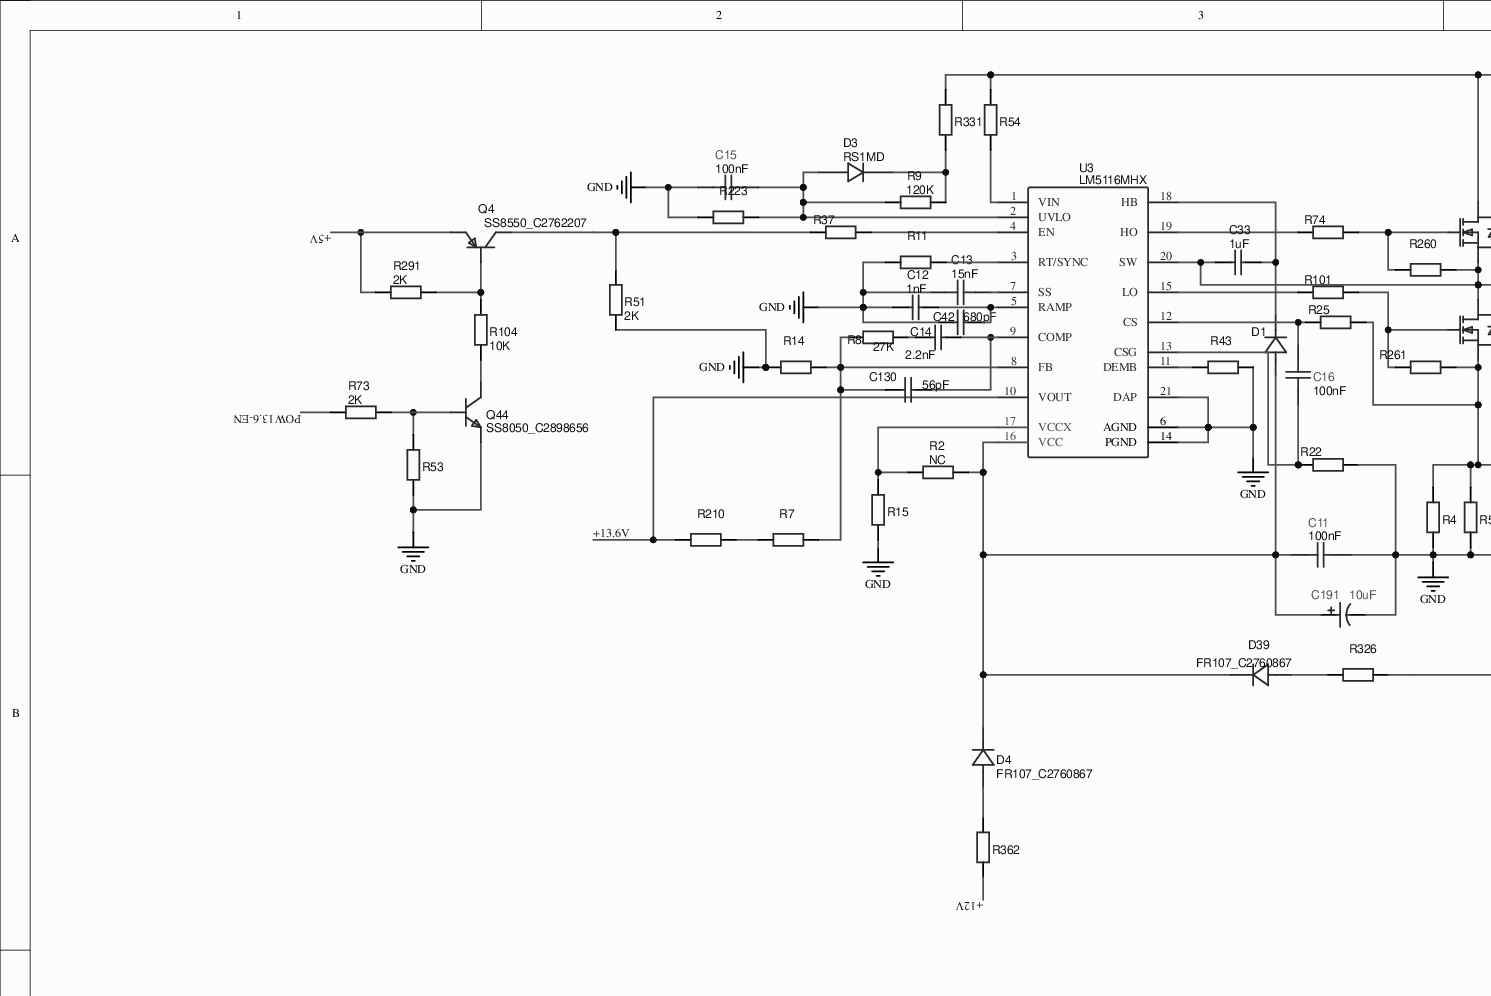
[diagram p0: MISC84402-12.SchDoc, top left]
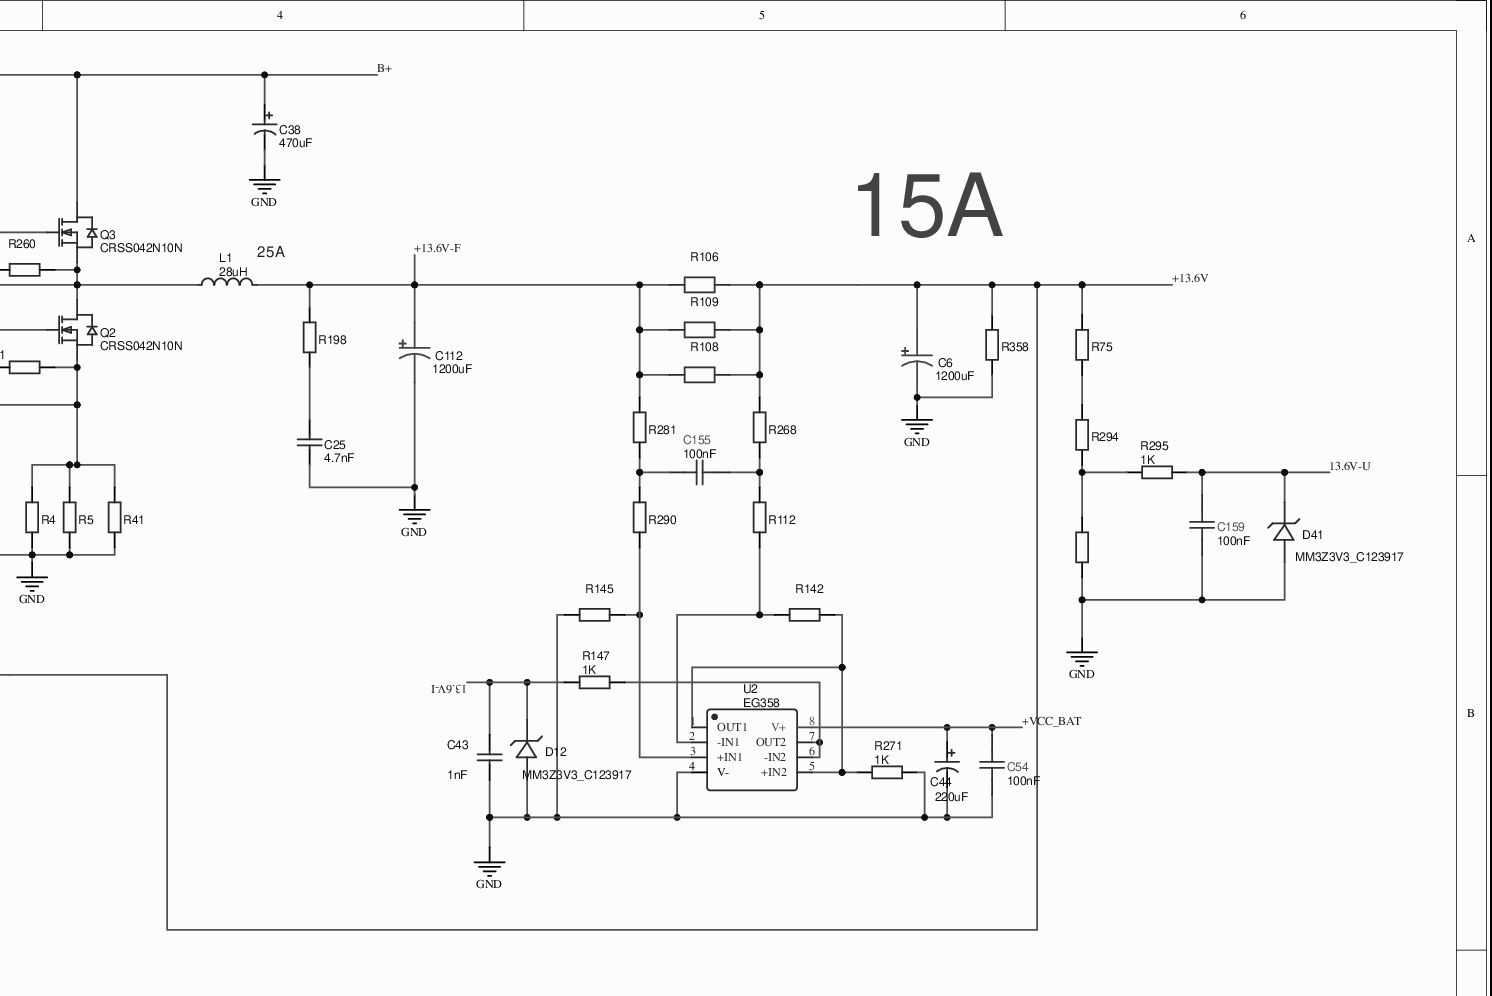
[diagram p1: MISC84402-12.SchDoc, top right]
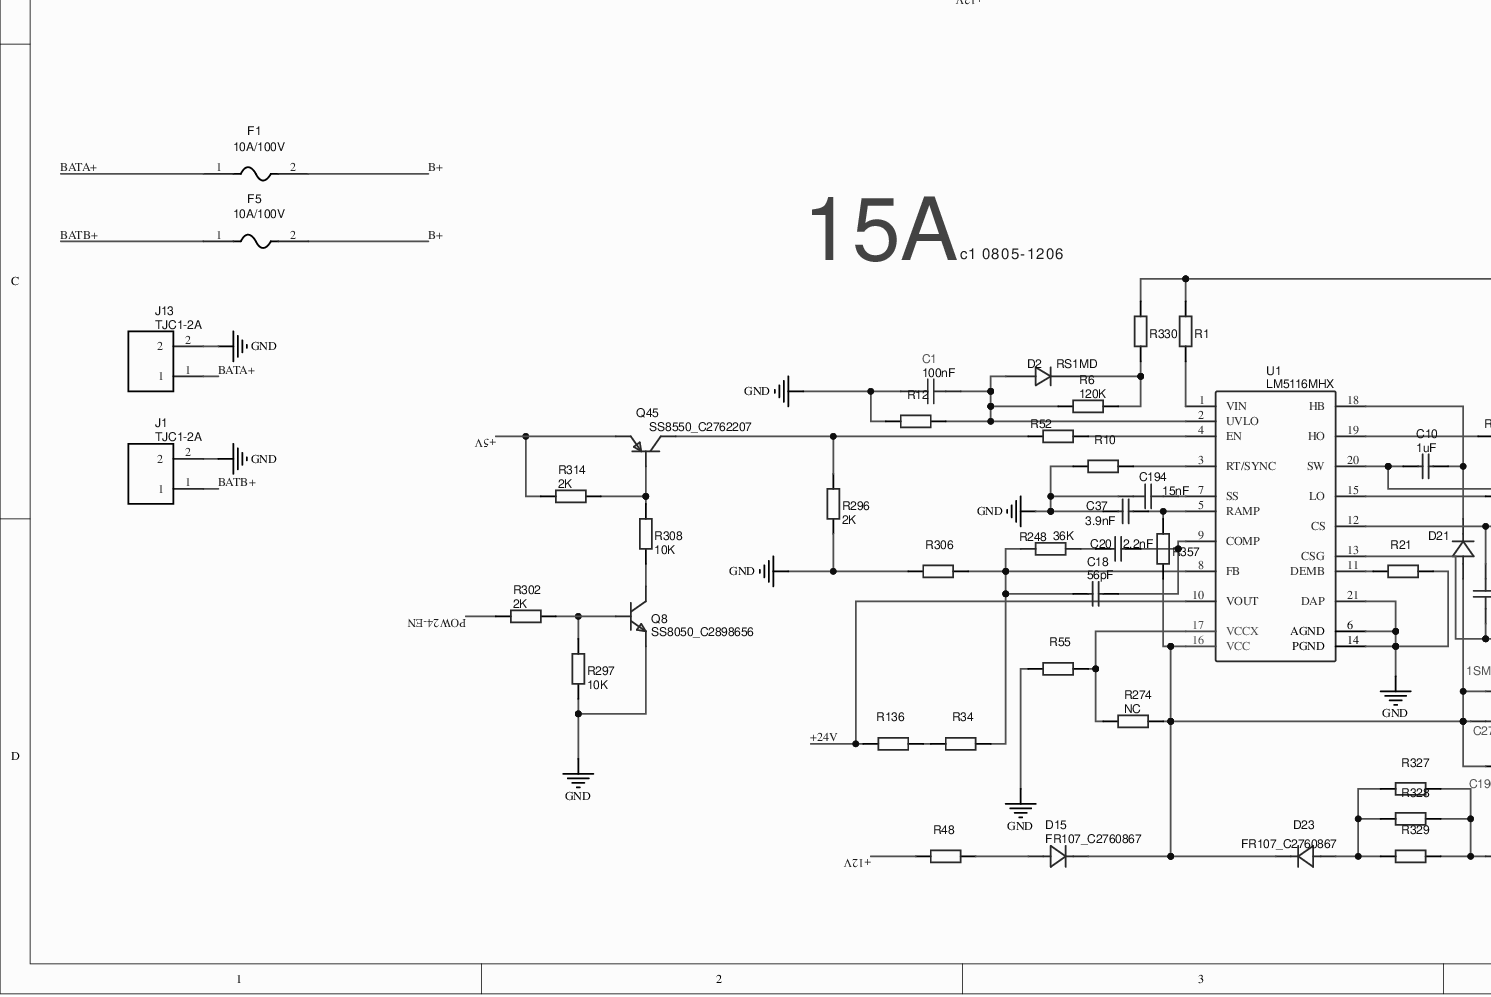
[diagram p2: MISC84402-12.SchDoc, bottom left]
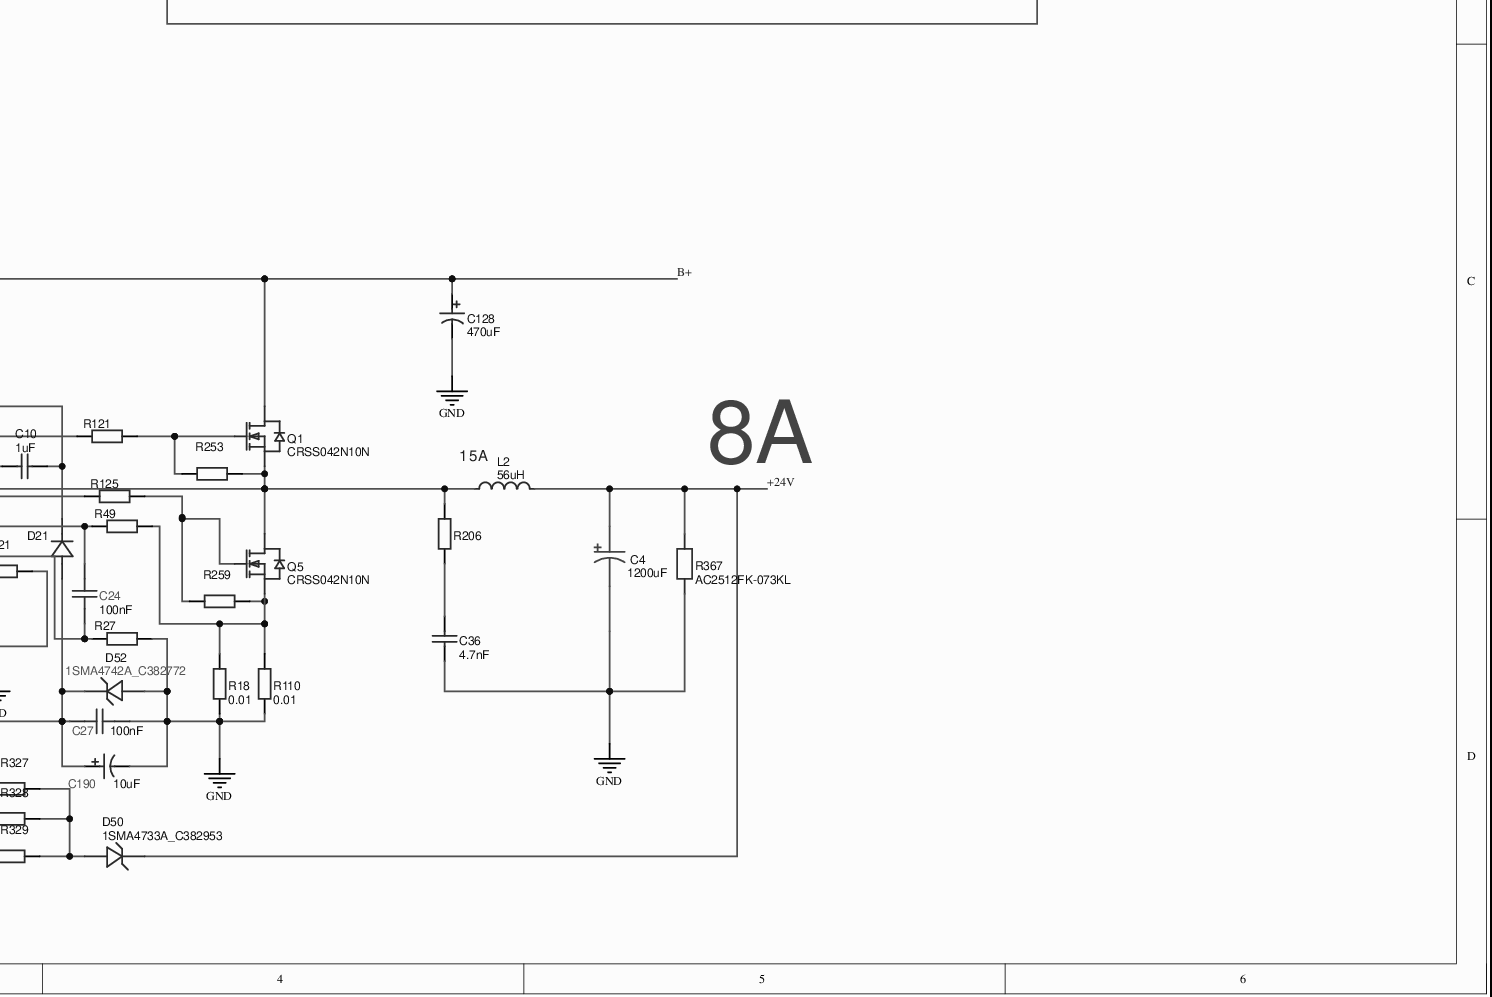
[diagram p3: MISC84402-12.SchDoc, bottom right]
# Altium project MISC84402-4.PrjPcb (part 4 of 7)

## Sheet MISC84402-12.SchDoc
size 488 x 321 mm

### Parts
C1  100nF  [C0603]
C4  1200uF  [CAP-TH_BD13.0-P5.00-D1.2-FD]
C6  1200uF  [CAP-TH_BD13.0-P5.00-D1.2-FD]
C10  1uF  [C0603]
C11  100nF  [C0603]
C12  1nF  [C0603]
C13  15nF  [C0603]
C14  2.2nF  [C0603]
C15  100nF  [C0603]
C16  100nF  [C0603]
C18  56pF  [C0603]
C20  2.2nF  [C0603]
C24  100nF  [C0603]
C25  4.7nF  [C1206]
C27  100nF  [C0603]
C33  1uF  [C0603]
C36  4.7nF  [C1206]
C37  3.9nF  [C0603]
C38  470uF  [CAP-TH_BD12.5-P5.00-D0.6-FD]
C42  680pF  [C0603]
C43  1nF  [C0603]
C44  220uF  [CAP-TH_BD6.3-P2.50-D1.0-FD]
C54  100nF  [C0603]
C112  1200uF  [CAP-TH_BD13.0-P5.00-D1.2-FD]
C128  470uF  [CAP-TH_BD12.5-P5.00-D0.6-FD]
C130  56pF  [C0603]
C155  100nF  [C0603]
C159  100nF  [C0603]
C190  10uF  [CAP-TH_BD5.0-P2.5-D0.5-FD]
C191  10uF  [CAP-TH_BD5.0-P2.5-D0.5-FD]
C194  15nF  [C0603]
D1  FR107_C2760867  [SOD-123FL_L2.7-W1.8-LS3.8-RD]  (value not drawn)
D2  RS1MD  [SMA_L4.3-W2.6-LS5.2-RD]
D3  RS1MD  [SMA_L4.3-W2.6-LS5.2-RD]
D4  FR107_C2760867  [SOD-123FL_L2.7-W1.8-LS3.8-RD]
D12  MM3Z3V3_C123917  [SOD-323_L1.8-W1.3-LS2.5-RD]
D15  FR107_C2760867  [SOD-123FL_L2.7-W1.8-LS3.8-RD]
D21  FR107_C2760867  [SOD-123FL_L2.7-W1.8-LS3.8-RD]  (value not drawn)
D23  FR107_C2760867  [SOD-123FL_L2.7-W1.8-LS3.8-RD]
D39  FR107_C2760867  [SOD-123FL_L2.7-W1.8-LS3.8-RD]
D41  MM3Z3V3_C123917  [SOD-323_L1.8-W1.3-LS2.5-RD]
D50  1SMA4733A_C382953  [SMA_L4.4-W2.6-LS5.0-RD]
D52  1SMA4742A_C382772  [SMA_L4.4-W2.6-LS5.0-RD]
F1  10A/100V  [FUSE-SMD_L6.1-W2.5]
F5  10A/100V  [FUSE-SMD_L6.1-W2.5]
J1  TJC1-2A  [CONN-TH_XT30UPB-F-W]
J13  TJC1-2A  [CONN-TH_XT30UPB-F-W]
L1  28uH  [IND-TH_CS270026-W280M-N]
L2  56uH  [IND-TH_CS270026-W560M-N]
Q1  CRSS042N10N  [TO-263-3_L10.2-W10.7-P5.08-LS16.2-TL]
Q2  CRSS042N10N  [TO-263-3_L10.2-W10.7-P5.08-LS16.2-TL]
Q3  CRSS042N10N  [TO-263-3_L10.2-W10.7-P5.08-LS16.2-TL]
Q4  SS8550_C2762207  [SOT-23-3_L2.9-W1.3-P1.90-LS2.4-BR]
Q5  CRSS042N10N  [TO-263-3_L10.2-W10.7-P5.08-LS16.2-TL]
Q8  SS8050_C2898656  [SOT-23-3_L2.9-W1.3-P1.90-LS2.4-BR]
Q44  SS8050_C2898656  [SOT-23-3_L2.9-W1.3-P1.90-LS2.4-BR]
Q45  SS8550_C2762207  [SOT-23-3_L2.9-W1.3-P1.90-LS2.4-BR]
R1  (no value)  [R1206]
R2  NC  [R0603]
R4  (no value)  [R2512]
R5  (no value)  [R2512]
R6  120K  [R0603]
R7  (no value)  [R0603]
R8  27K  [R0603]
R9  120K  [R0603]
R10  (no value)  [R0603]
R11  (no value)  [R0603]
R12  (no value)  [R0603]
R14  (no value)  [R0603]
R15  (no value)  [R0603]
R18  0.01  [R2512]
R21  (no value)  [R0603]
R22  (no value)  [R0603]
R25  (no value)  [R0603]
R27  (no value)  [R0603]
R34  (no value)  [R0603]
R37  (no value)  [R0603]
R41  (no value)  [R2512]
R43  (no value)  [R0603]
R48  (no value)  [R0603]
R49  (no value)  [R0603]
R51  2K  [R0603]
R52  (no value)  [R0603]
R53  (no value)  [R0603]
R54  (no value)  [R1206]
R55  (no value)  [R0603]
R73  2K  [R0603]
R74  (no value)  [R0805]
R75  (no value)  [R0603]
R101  (no value)  [R0805]
R104  10K  [R0603]
R106  (no value)  [R2512]
R107  (no value)  [R0603]
R108  (no value)  [R2512]
R109  (no value)  [R2512]
R110  0.01  [R2512]
R112  (no value)  [R0603]
R121  (no value)  [R0805]
R125  (no value)  [R0805]
R136  (no value)  [R0603]
R142  (no value)  [R0603]
R145  (no value)  [R0603]
R147  1K  [R0603]
R198  (no value)  [R1206]
R206  (no value)  [R1206]
R210  (no value)  [R0603]
R223  (no value)  [R0603]
R248  36K  [R0603]
R253  (no value)  [R0603]
R259  (no value)  [R0603]
R260  (no value)  [R0603]
R261  (no value)  [R0603]
R268  (no value)  [R0603]
R271  1K  [R0603]
R274  NC  [R0603]
R281  (no value)  [R0603]
R290  (no value)  [R0603]
R291  2K  [R0603]
R294  (no value)  [R0603]
R295  1K  [R0603]
R296  2K  [R0603]
R297  10K  [R0603]
R302  2K  [R0603]
R306  (no value)  [R0603]
R308  10K  [R0603]
R314  2K  [R0603]
R326  (no value)  [R0603]
R327  (no value)  [R0805]
R328  (no value)  [R0805]
R329  (no value)  [R0805]
R330  (no value)  [R1206]
R331  (no value)  [R1206]
R357  (no value)  [R0603]
R358  (no value)  [R2512]
R362  (no value)  [R0603]
R367  AC2512FK-073KL  [R2512]
U1  LM5116MHX  [HTSSOP-20_L6.5-W4.4-P0.65-LS6.4-BL-EP]
U2  EG358  [SOIC-8_L5.0-W4.0-P1.27-LS6.0-BL]
U3  LM5116MHX  [HTSSOP-20_L6.5-W4.4-P0.65-LS6.4-BL-EP]

### Nets
GND: C1.2 C4.2 C6.2 C11.1 C12.1 C13.2 C15.2 C25.1 C27.1 C36.1 C37.2 C38.2 C42.1 C43.1 C44.2 C54.2 C112.2 C128.2 C159.2 C190.2 C191.2 C194.2 D12.2(A) D41.2(A) D52.2(A) J1.2 J13.2 Q8.2(E) Q44.2(E) R4.1 R5.1 R10.1 R11.1 R12.1 R14.2 R15.1 R18.1 R21.2 R22.1 R27.1 R41.1 R43.2 R51.1 R53.2 R55.1 R107.1 R110.1 R145.1 R223.1 R271.2 R296.1 R297.2 R306.2 R358.1 R367.1 U1.6(AGND) U1.14(PGND) U1.21(DAP) U2.4(V-) U3.6(AGND) U3.14(PGND) U3.21(DAP)
13.6V-I: C43.2 D12.1(K) R147.2
13.6V-U: C159.1 D41.1(K) R295.1
+5V: Q4.2(E) Q45.2(E) R291.1 R314.1
+12V: R48.2 R362.1
+13.6V: C6.1 R75.2 R106.2 R108.2 R109.2 R210.1 R268.1 R326.2 R358.2 U3.10(VOUT)
+13.6V-F: C112.1 L1.2 R106.1 R108.1 R109.1 R198.2 R281.1
+24V: C4.1 D50.1(C) L2.2 R136.2 R367.2 U1.10(VOUT)
+VCC_BAT: C44.1 C54.1 U2.8(V+)
B+: C38.1 C128.1 F1.2 F5.2 Q1.2(D) Q3.2(D) R1.2 R54.2 R330.2 R331.2
BATA+: F1.1 J13.1
BATB+: F5.1 J1.1
POW13.6-EN: R73.1
POW24-EN: R302.1
NetC1_1: C1.1 D2.2 R6.1 R12.2 U1.2(UVLO)
NetC10_1: C10.1 L2.1 Q1.3(S) Q5.2(D) R206.2 R253.1 U1.20(SW)
NetC10_2: C10.2 D21.1(K) U1.18(HB)
NetC11_2: C11.2 C191.1 D1.2(A) D4.1(K) D39.1(K) R2.2 U3.16(VCC)
NetC12_2: C12.2 C42.2 U3.5(RAMP)
NetC13_1: C13.1 U3.7(SS)
NetC14_1: C14.1 R8.2
NetC14_2: C14.2 C130.1 U3.9(COMP)
NetC15_1: C15.1 D3.2 R9.1 R223.2 U3.2(UVLO)
NetC16_1: C16.1 R25.2 U3.12(CS)
NetC16_2: C16.2 R22.2 U3.13(CSG)
NetC18_1: C18.1 C20.1 U1.9(COMP)
NetC18_2: C18.2 R34.2 R248.1 R306.1 U1.8(FB)
NetC20_2: C20.2 R248.2
NetC24_1: C24.1 R49.2 U1.12(CS)
NetC24_2: C24.2 R27.2 U1.13(CSG)
NetC25_2: C25.2 R198.1
NetC27_2: C27.2 C190.1 D15.1(K) D21.2(A) D23.1(K) D52.1(C) R274.2 R357.1 U1.16(VCC)
NetC33_1: C33.1 L1.1 Q2.2(D) Q3.3(S) R260.1 U3.20(SW)
NetC33_2: C33.2 D1.1(K) U3.18(HB)
NetC36_2: C36.2 R206.1
NetC37_1: C37.1 R357.2 U1.5(RAMP)
NetC130_2: C130.2 R7.2 R8.1 R14.1 U3.8(FB)
NetC155_1: C155.1 R112.1 R268.2
NetC155_2: C155.2 R281.2 R290.1
NetC194_1: C194.1 U1.7(SS)
NetD2_1: D2.1 R6.2 R330.1
NetD3_1: D3.1 R9.2 R331.1
NetD4_2: D4.2(A) R362.2
NetD15_2: D15.2(A) R48.1
NetD23_2: D23.2(A) R327.1 R328.1 R329.1
NetD39_2: D39.2(A) R326.1
NetD50_2: D50.2(A) R327.2 R328.2 R329.2
NetQ1_1: Q1.1(G) R121.1 R253.2
NetQ2_1: Q2.1(G) R101.1 R261.2
NetQ2_3: Q2.3(S) R4.2 R5.2 R25.1 R41.2 R261.1
NetQ3_1: Q3.1(G) R74.1 R260.2
NetQ4_1: Q4.1(B) R104.2 R291.2
NetQ4_3: Q4.3(C) R37.1 R51.2
NetQ5_1: Q5.1(G) R125.1 R259.2
NetQ5_3: Q5.3(S) R18.2 R49.1 R110.2 R259.1
NetQ8_1: Q8.1(B) R297.1 R302.2
NetQ8_3: Q8.3(C) R308.1
NetQ44_1: Q44.1(B) R53.1 R73.2
NetQ44_3: Q44.3(C) R104.1
NetQ45_1: Q45.1(B) R308.2 R314.2
NetQ45_3: Q45.3(C) R52.1 R296.2
NetR1_1: R1.1 U1.1(VIN)
NetR2_1: R2.1 R15.2 U3.17(VCCX)
NetR7_1: R7.1 R210.2
NetR10_2: R10.2 U1.3(RT/SYNC)
NetR11_2: R11.2 U3.3(RT/SYNC)
NetR21_1: R21.1 U1.11(DEMB)
NetR34_1: R34.1 R136.1
NetR37_2: R37.2 U3.4(EN)
NetR43_1: R43.1 U3.11(DEMB)
NetR52_2: R52.2 U1.4(EN)
NetR54_1: R54.1 U3.1(VIN)
NetR55_2: R55.2 R274.1 U1.17(VCCX)
NetR74_2: R74.2 U3.19(HO)
NetR75_1: R75.1 R294.2
NetR101_2: R101.2 U3.15(LO)
NetR107_2: R107.2 R294.1 R295.2
NetR112_2: R112.2 R142.1 U2.2(-IN1)
NetR121_2: R121.2 U1.19(HO)
NetR125_2: R125.2 U1.15(LO)
NetR142_2: R142.2 R271.1 U2.1(OUT1) U2.5(+IN2)
NetR145_2: R145.2 R290.2 U2.3(+IN1)
NetR147_1: R147.1 U2.6(-IN2) U2.7(OUT2)

### Notes on the sheet
- (near L1) 25A
- 15A
- c1 0805-1206
- (near L2) 15A
- 8A

### Library data of the parts
C1 C11 C15 C16 C24 C27 C54 C155 C159 = 100nF: BOM_Manufacturer: SAMSUNG; BOM_Manufacturer Part: CL10B104KC8NNNC; nameAlias: Capacitance; BOM_Supplier: LCSC; BOM_Supplier Part: C15725; BOM_JLCPCB Part Class: Extended Part; spicePre: C; spiceSymbolName: CL10B104KC8NNNC
C4 C6 C112 = 1200uF: BOM_Manufacturer: CapXon; BOM_Manufacturer Part: GF122M025I200A; nameAlias: Capacitance; BOM_Supplier: LCSC; BOM_Supplier Part: C89779; BOM_JLCPCB Part Class: Extended Part; spicePre: C; spiceSymbolName: GF122M025I200A
C10 C33 = 1uF: BOM_Manufacturer Part: CL10A105KB8NNNC; BOM_Manufacturer: SAMSUNG; nameAlias: Capacitance; BOM_Supplier: LCSC; BOM_Supplier Part: C15849; BOM_JLCPCB Part Class: Basic Part; spicePre: C; spiceSymbolName: CL10A105KB8NNNC
C12 C43 = 1nF: BOM_Manufacturer Part: CL10B102KB8NNNC; BOM_Manufacturer: SAMSUNG; nameAlias: Capacitance; BOM_Supplier: LCSC; BOM_Supplier Part: C1588; BOM_JLCPCB Part Class: Basic Part; spicePre: C; spiceSymbolName: CL10B102KB8NNNC
C13 C194 = 15nF: BOM_Manufacturer: Walsin Tech Corp; BOM_Manufacturer Part: 0603B153K500CT; nameAlias: Capacitance; Contributor: LCSC; BOM_Supplier: LCSC; BOM_Supplier Part: C296018; spicePre: C; spiceSymbolName: 0603B153K500CT
C14 = 2.2nF: BOM_Manufacturer: YAGEO; BOM_Manufacturer Part: CC0603KRX7R9BB222; nameAlias: Capacitance; BOM_Supplier: LCSC; BOM_Supplier Part: C107082; BOM_JLCPCB Part Class: Extended Part; spicePre: C; spiceSymbolName: CC0603KRX7R9BB222
C18 C130 = 56pF: BOM_Manufacturer Part: CL10C560JB8NNNC; BOM_Manufacturer: SAMSUNG; nameAlias: Capacitance; BOM_Supplier: LCSC; BOM_Supplier Part: C39148; BOM_JLCPCB Part Class: Basic Part; spicePre: C; spiceSymbolName: CL10C560JB8NNNC
C20 = 2.2nF: BOM_Manufacturer Part: CL10B222KB8NNNC; BOM_Manufacturer: SAMSUNG; nameAlias: Capacitance; BOM_Supplier: LCSC; BOM_Supplier Part: C16033; BOM_JLCPCB Part Class: Extended Part; spicePre: C; spiceSymbolName: CL10B222KB8NNNC
C25 C36 = 4.7nF: BOM_Manufacturer: FH; BOM_Manufacturer Part: 1206B472K102NT; nameAlias: Capacitance; BOM_Supplier: LCSC; BOM_Supplier Part: C9192; BOM_JLCPCB Part Class: Extended Part; spicePre: C; spiceSymbolName: 1206B472K102NT
C37 = 3.9nF: BOM_Manufacturer: FH; BOM_Manufacturer Part: 0603B392K500NT; nameAlias: Capacitance; BOM_Supplier: LCSC; BOM_Supplier Part: C1618; BOM_JLCPCB Part Class: Extended Part; spicePre: C; spiceSymbolName: 0603B392K500NT
C38 C128 = 470uF: BOM_Manufacturer: ValuePro; nameAlias: Capacitance; BOM_Supplier: LCSC; BOM_Supplier Part: C18823; BOM_JLCPCB Part Class: Extended Part; spicePre: C
C42 = 680pF: BOM_Manufacturer: FH; BOM_Manufacturer Part: 0603B681K500NT; nameAlias: Capacitance; BOM_Supplier: LCSC; BOM_Supplier Part: C1630; BOM_JLCPCB Part Class: Basic Part; spicePre: C; spiceSymbolName: 0603B681K500NT
C44 = 220uF: BOM_Manufacturer: ValuePro; BOM_Manufacturer Part: 220uF 16V 6.3*11; nameAlias: Capacitance; BOM_Supplier: LCSC; BOM_Supplier Part: C43349; BOM_JLCPCB Part Class: Extended Part; spicePre: C; spiceSymbolName: 220uF 16V 6.3*11
C190 C191 = 10uF: BOM_Manufacturer Part: C10uF63V2.5mm5x11mm; BOM_Manufacturer: ReliaPro; nameAlias: Capacitance; BOM_Supplier: LCSC; BOM_Supplier Part: C32455; BOM_JLCPCB Part Class: Extended Part; spicePre: C; spiceSymbolName: C10uF63V2.5mm5x11mm
D1 D4 D15 D23 D39 = FR107_C2760867: BOM_Manufacturer Part: FR107; Contributor: LCSC; BOM_Supplier: LCSC; BOM_Supplier Part: C2760867; BOM_JLCPCB Part Class: Extended Part; spicePre: D; spiceSymbolName: FR107_C2760867
D2 D3 = RS1MD: BOM_Manufacturer: SEMTECH; BOM_Supplier: LCSC; BOM_Manufacturer Part: RS1MD; BOM_Supplier Part: C84509; BOM_JLCPCB Part Class: Extended Part; spicePre: D; spiceSymbolName: RS1MD
D12 D41 = MM3Z3V3_C123917: BOM_Manufacturer: Shandong Jingdao Microelectronics; Contributor: LCSC; BOM_Supplier: LCSC; BOM_Supplier Part: C123917; BOM_Manufacturer Part: MM3Z3V3; BOM_JLCPCB Part Class: Extended Part; spicePre: D; spiceSymbolName: MM3Z3V3_C123917
D21 = FR107_C2760867: BOM_Manufacturer Part: FR107; Contributor: LCSC; Package Display: No; BOM_Supplier: LCSC; BOM_Supplier Part: C2760867; BOM_JLCPCB Part Class: Extended Part; spicePre: D; spiceSymbolName: FR107_C2760867
D50 = 1SMA4733A_C382953: BOM_Manufacturer: Shandong Jingdao Microelectronics; Contributor: LCSC; BOM_Supplier: LCSC; BOM_Supplier Part: C382953; BOM_Manufacturer Part: 1SMA4733A; BOM_JLCPCB Part Class: Extended Part; spicePre: D; spiceSymbolName: 1SMA4733A_C382953
D52 = 1SMA4742A_C382772: BOM_Manufacturer: Shandong Jingdao Microelectronics; Contributor: LCSC; BOM_Supplier: LCSC; BOM_Supplier Part: C382772; BOM_Manufacturer Part: 1SMA4742A; BOM_JLCPCB Part Class: Extended Part; spicePre: D; spiceSymbolName: 1SMA4742A_C382772
F1 F5 = 10A/100V: BOM_Manufacturer: RUILON; BOM_Supplier: LCSC; BOM_Supplier Part: C30198; BOM_JLCPCB Part Class: Extended Part; spicePre: F
J1 J13 = TJC1-2A: BOM_Manufacturer: ReliaPro; BOM_Supplier: LCSC; BOM_Manufacturer Part: TJC1-2A; BOM_Supplier Part: C29632; spicePre: J; spiceSymbolName: TJC1-2A
L1 = 28uH: nameAlias: Value(H); Contributor: LCEDA_Lib; spicePre: L; spiceSymbolName: L0603_US
L2 = 56uH: nameAlias: Value(H); Contributor: LCEDA_Lib; spicePre: L; spiceSymbolName: L0603_US
Q1-Q3 Q5 = CRSS042N10N: BOM_Manufacturer: CRMICRO; Contributor: LCSC; BOM_Supplier: LCSC; BOM_Supplier Part: C410926; BOM_Manufacturer Part: CRSS042N10N; BOM_JLCPCB Part Class: Extended Part; spicePre: Q; spiceSymbolName: CRSS042N10N
Q4 Q45 = SS8550_C2762207: BOM_Manufacturer Part: SS8550; Contributor: LCSC; BOM_Supplier: LCSC; BOM_Supplier Part: C2762207; BOM_JLCPCB Part Class: Extended Part; spicePre: Q; spiceSymbolName: SS8550_C2762207
Q8 Q44 = SS8050_C2898656: BOM_Manufacturer Part: SS8050; Contributor: LCSC; BOM_Supplier: LCSC; BOM_Supplier Part: C2898656; spicePre: Q; spiceSymbolName: SS8050_C2898656
R1 R54 R330 R331 = (no symbol name): BOM_Manufacturer: UniOhm; BOM_Manufacturer Part: 1206W4F100JT5E; nameAlias: Resistance; Resistance (Ohms): 10; BOM_Supplier: LCSC; BOM_Supplier Part: C17903; BOM_JLCPCB Part Class: Basic Part; spicePre: R; spiceSymbolName: 1206W4F100JT5E
R2 R274 = NC: BOM_Manufacturer: UniOhm; BOM_Manufacturer Part: 0603WAF0000T5E; nameAlias: Resistance; Resistance (Ohms): 0; BOM_Supplier: LCSC; BOM_Supplier Part: C21189; BOM_JLCPCB Part Class: Basic Part; spicePre: R; spiceSymbolName: 0603WAF0000T5E
R4 R5 R41 = (no symbol name): BOM_Manufacturer: PSA; BOM_Manufacturer Part: FMF25FPJR015-LHL; nameAlias: Resistance; Resistance (Ohms): 0.015; BOM_Supplier: LCSC; BOM_Supplier Part: C105381; BOM_JLCPCB Part Class: Extended Part; spicePre: R; spiceSymbolName: FMF25FPJR015-LHL
R6 R9 = 120K: BOM_Manufacturer: YAGEO; BOM_Manufacturer Part: RC0603FR-07120KL; nameAlias: Resistance (Ohms); BOM_Supplier: LCSC; BOM_Supplier Part: C114607; BOM_JLCPCB Part Class: Extended Part; spicePre: R; spiceSymbolName: RC0603FR-07120KL
R7 = (no symbol name): BOM_Manufacturer: UniOhm; BOM_Manufacturer Part: 0603WAF1802T5E; nameAlias: Resistance; Resistance (Ohms): 18K; BOM_Supplier: LCSC; BOM_Supplier Part: C25810; BOM_JLCPCB Part Class: Basic Part; spicePre: R; spiceSymbolName: 0603WAF1802T5E
R8 = 27K: BOM_Manufacturer: FH; BOM_Manufacturer Part: RS-03K273JT; nameAlias: Resistance (Ohms); BOM_Supplier: LCSC; BOM_Supplier Part: C73798; spicePre: R; spiceSymbolName: RS-03K273JT
R10 R11 = (no symbol name): BOM_Manufacturer: UniOhm; BOM_Manufacturer Part: 0603WAF7502T5E; nameAlias: Resistance; Resistance (Ohms): 75K; BOM_Supplier: LCSC; BOM_Supplier Part: C23242; BOM_JLCPCB Part Class: Basic Part; spicePre: R; spiceSymbolName: 0603WAF7502T5E
R12 R223 = (no symbol name): BOM_Manufacturer Part: 0603WAF5101T5E; BOM_Manufacturer: UniOhm; Resistance (Ohms): 5.1K; nameAlias: Resistance; BOM_Supplier: LCSC; BOM_Supplier Part: C23186; BOM_JLCPCB Part Class: Basic Part; spicePre: R; spiceSymbolName: 0603WAF5101T5E
R14 R306 = (no symbol name): BOM_Manufacturer: UniOhm; BOM_Manufacturer Part: 0603WAF2001T5E; nameAlias: Resistance; Resistance (Ohms): 2K; BOM_Supplier: LCSC; BOM_Supplier Part: C22975; BOM_JLCPCB Part Class: Basic Part; spicePre: R; spiceSymbolName: 0603WAF2001T5E
R15 R37 R52 R55 R294 = (no symbol name): BOM_Manufacturer: UniOhm; BOM_Manufacturer Part: 0603WAF0000T5E; nameAlias: Resistance; Resistance (Ohms): 0; BOM_Supplier: LCSC; BOM_Supplier Part: C21189; BOM_JLCPCB Part Class: Basic Part; spicePre: R; spiceSymbolName: 0603WAF0000T5E
R18 R110 = 0.01: BOM_Manufacturer Part: MRF6432(2512)LR010JTS; BOM_Manufacturer: SUP; BOM_Supplier Part: C76272; BOM_Supplier: LCSC; BOM_JLCPCB Part Class: Extended Part; spicePre: R; spiceSymbolName: MRF6432(2512)LR010JTS
R21 R43 R53 R107 = (no symbol name): BOM_Manufacturer: UniOhm; BOM_Manufacturer Part: 0603WAF1002T5E; nameAlias: Resistance; Resistance (Ohms): 10K; BOM_Supplier: LCSC; BOM_Supplier Part: C25804; BOM_JLCPCB Part Class: Basic Part; spicePre: R; spiceSymbolName: 0603WAF1002T5E
R22 R25 R27 R49 R268 R281 = (no symbol name): BOM_Manufacturer: UniOhm; BOM_Manufacturer Part: 0603WAF100KT5E; nameAlias: Resistance; Resistance (Ohms): 1; BOM_Supplier: LCSC; BOM_Supplier Part: C22936; BOM_JLCPCB Part Class: Basic Part; spicePre: R; spiceSymbolName: 0603WAF100KT5E